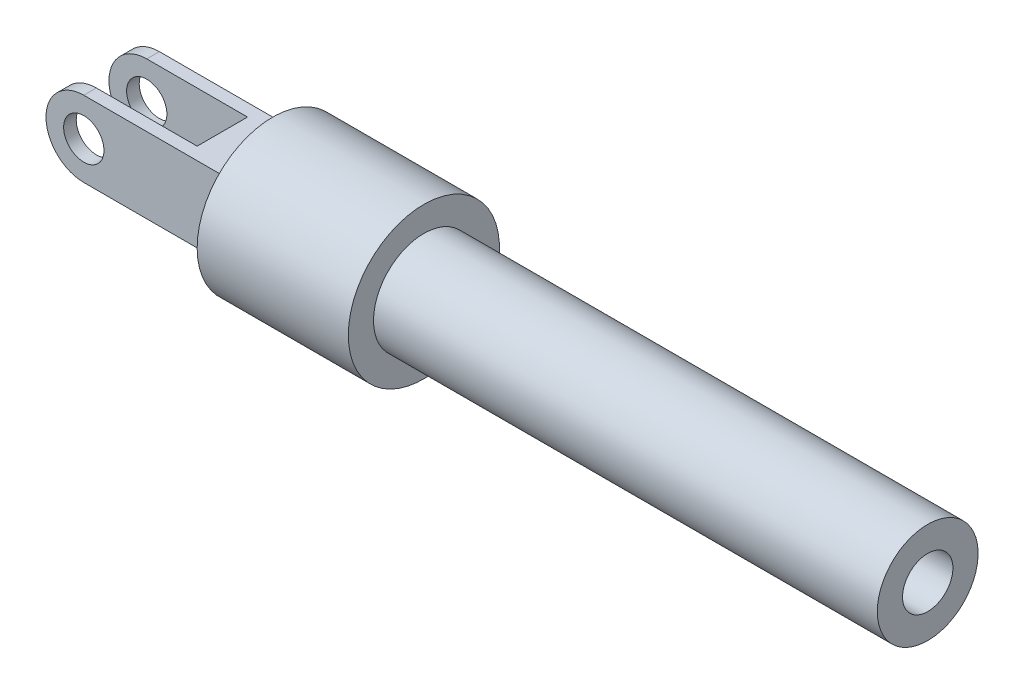
from build123d import *

# Parameters (mm, degrees)
SKETCH2_R           = 0.4
BOSS_EXTRUDE1_DEPTH = 0.75
CUT_EXTRUDE1_DEPTH  = 0.5
SKETCH4_R           = 0.5
CUT_EXTRUDE2_DEPTH  = 6


with BuildPart() as part:
    # Sketch1 → Revolve1 (revolve)
    with BuildSketch(Plane.XY, mode=Mode.PRIVATE) as revolve1_sk:
        Polygon((0, 0), (0, 1.5), (3, 1.5), (3, 1), (13, 1), (13, 0), align=None)
    revolve(revolve1_sk.sketch.rotate(Axis((0.124352332, 0, 0), (1, 0, 0)), 90), axis=Axis((0.124352332, 0, 0), (1, 0, 0)))

    # Sketch2 → Boss-Extrude1 (add, symmetric)
    with BuildSketch(Plane.XY):
        with BuildLine():
            Line((0, 0.75), (0, -0.75))
            Line((0, -0.75), (-3, -0.75))
            ThreePointArc((-3, -0.75), (-3.75, 0), (-3, 0.75))
            Line((-3, 0.75), (0, 0.75))
        make_face()
        with Locations((-3, 0)):
            Circle(SKETCH2_R, mode=Mode.SUBTRACT)
    extrude(amount=BOSS_EXTRUDE1_DEPTH, both=True)

    # Sketch3 → Cut-Extrude1 (cut, symmetric)
    with BuildSketch(Plane.XY):
        with BuildLine():
            Line((-1, 0.75), (-1, -0.75))
            Line((-1, -0.75), (-3, -0.75))
            ThreePointArc((-3, -0.75), (-3.75, 0), (-3, 0.75))
            Line((-3, 0.75), (-1, 0.75))
        make_face()
    extrude(amount=CUT_EXTRUDE1_DEPTH, both=True, mode=Mode.SUBTRACT)

    # Sketch4 → Cut-Extrude2 (cut)
    with BuildSketch(Plane(origin=(13, 0, 0), x_dir=(0, 0, -1), z_dir=(1, 0, 0))):
        Circle(SKETCH4_R)
    extrude(amount=-CUT_EXTRUDE2_DEPTH, mode=Mode.SUBTRACT)


solid = part.part
